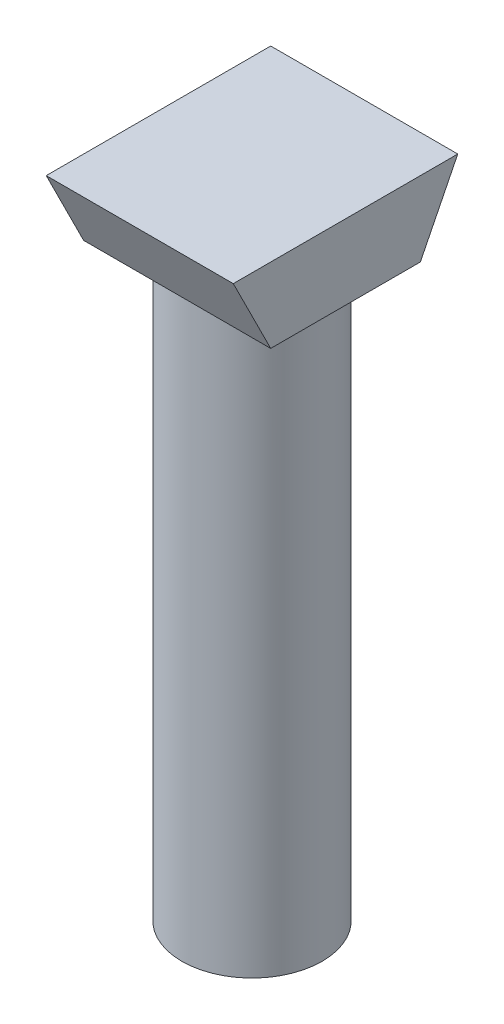
from build123d import *

# Parameters (mm, degrees)
SKETCH1_W               = 48
SKETCH1_H               = 16
BOSS_EXTRUDE1_DEPTH     = 20
CUT_EXTRUDE1_DEPTH      = 33.249030993
CUT_EXTRUDE1_DEPTH_BACK = 33.249030993
SKETCH3_R               = 15
BOSS_EXTRUDE2_DEPTH     = 124


with BuildPart() as part:
    # Sketch1 → Boss-Extrude1 (new, symmetric)
    with BuildSketch(Plane(origin=(0, 0, 0), x_dir=(0, 0, -1), z_dir=(1, 0, 0))):
        Rectangle(SKETCH1_W, SKETCH1_H)
    extrude(amount=BOSS_EXTRUDE1_DEPTH, both=True)

    # Sketch2 → Cut-Extrude1 (cut, two sides: drawn at the far end of the back side and taken through both)
    with BuildSketch(Plane(origin=(0, 0, 0), x_dir=(0, 0, -1), z_dir=(1, 0, 0)).offset(-CUT_EXTRUDE1_DEPTH_BACK)):
        Polygon((-24, 8), (-16, -8), (-24, -8), align=None)
        Polygon((24, 8), (24, -8), (16, -8), align=None)
    extrude(amount=CUT_EXTRUDE1_DEPTH + CUT_EXTRUDE1_DEPTH_BACK, mode=Mode.SUBTRACT)

    # Sketch3 → Boss-Extrude2 (add)
    with BuildSketch(Plane.XZ.offset(8)):
        with Locations(Location((0, 0, 0), (0, 0, 90))):
            Circle(SKETCH3_R)
    extrude(amount=BOSS_EXTRUDE2_DEPTH)


solid = part.part
